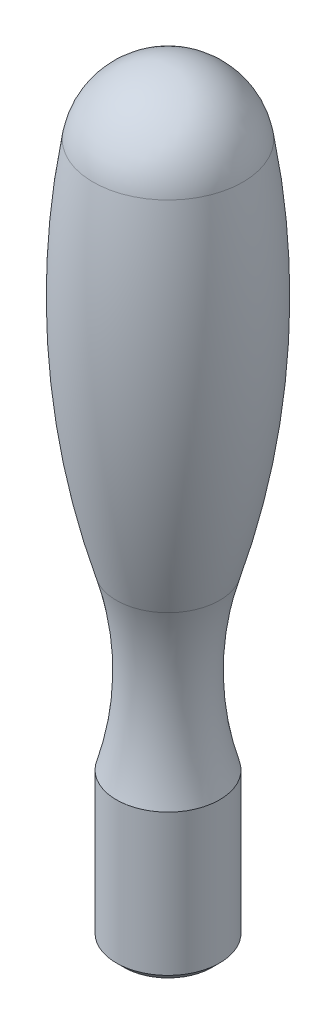
SolidWorks part; units mm, degrees
ref_plane "Front Plane" through (0, 0, 0) normal (0, 0, 1) x (1, 0, 0)
ref_plane "Top Plane" through (0, 0, 0) normal (0, 1, 0) x (1, 0, 0)
ref_plane "Right Plane" through (0, 0, 0) normal (1, 0, 0) x (0, 0, -1)
sketch "Sketch1" plane through (0, 0, 0) normal (0, 0, 1) x (1, 0, 0)
  line L0 (-106.5, 85.3) -> (-106.5, 109.5772) construction
  line L1 (-103.1, 87.263) -> (-103.1, 97.0767) construction
  line L2 (-103.1, 87.763) -> (-103.1, 97.0767)
  line L3 (-106.5, 137.263) -> (-106.5, 87.263)
  line L4 (-103.1, 87.263) -> (-109.9, 87.263) construction
  line L5 (-106.5, 87.263) -> (-103.6, 87.263)
  line L6 (-103.6, 87.263) -> (-103.1, 87.763)
  line L7 (-103.1, 97.0767) -> (-103.1, 130.8697) construction
  arc A1 (-101.5671, 133.0797) -> (-106.5, 137.263) centre (-106.5, 132.263) ccw
  arc A2 (-103.1, 108.4534) -> (-103.1, 97.0767) centre (-83.926, 102.7651) ccw
  arc A3 (-101.5671, 133.0797) -> (-103.1, 108.4534) centre (-155.8285, 124.0963) cw
  circle A4 centre (-106.5, 71.3) radius 26 construction
  point P5 (-103.1, 87.263)
  dimension "D1" = 5
  dimension "D3" = 55
  dimension "D4" = 20
  dimension "D2" = 50
revolve "Revolve1" add sketch "Sketch1" angle 360 about L0
